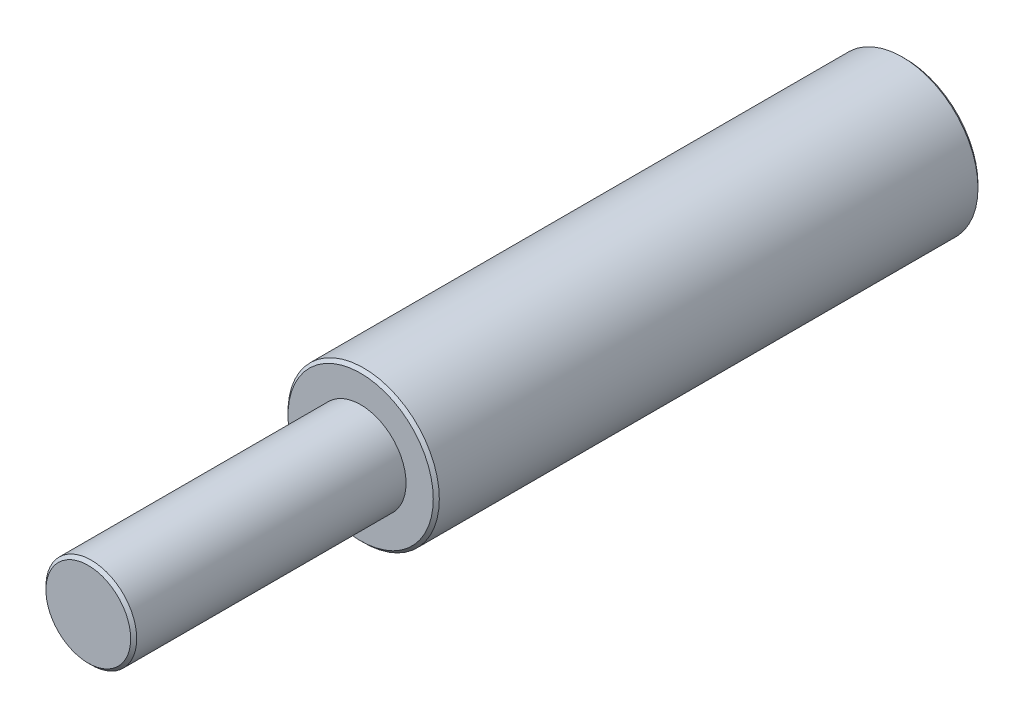
from build123d import *

# Parameters (mm, degrees)
SKETCH1_R           = 25
BOSS_EXTRUDE1_DEPTH = 180
SKETCH2_R           = 15
BOSS_EXTRUDE2_DEPTH = 90
CUT_EXTRUDE1_START  = -20
CUT_EXTRUDE1_DEPTH  = 120
CHAMFER1_SIZE       = 1
CUT_EXTRUDE2_START  = -10
SKETCH4_R           = 2.5
CUT_EXTRUDE2_DEPTH  = 10


with BuildPart() as part:
    # Sketch1 → Boss-Extrude1 (new body)
    with BuildSketch(Plane.XY):
        with Locations(Location((0, 0, 0), (0, 0, 180))):
            Circle(SKETCH1_R)
    extrude(amount=BOSS_EXTRUDE1_DEPTH)

    # Sketch2 → Boss-Extrude2 (add)
    with BuildSketch(Plane.XY.offset(180)):
        with Locations(Location((0, 0, 0), (0, 0, 180))):
            Circle(SKETCH2_R)
    extrude(amount=BOSS_EXTRUDE2_DEPTH)

    # Sketch3 → Cut-Extrude1 (cut)
    with BuildSketch(Plane(origin=(0, 0, 0), x_dir=(1, 0, 0), z_dir=(0, 1, 0)).offset(CUT_EXTRUDE1_START)):
        with BuildLine():
            Line((6, -84.229937471), (6, -134.229937471))
            ThreePointArc((6, -134.229937471), (0, -140.229937471), (-6, -134.229937471))
            Line((-6, -134.229937471), (-6, -84.229937471))
            ThreePointArc((-6, -84.229937471), (0, -78.229937471), (6, -84.229937471))
        make_face()
    extrude(amount=-CUT_EXTRUDE1_DEPTH, mode=Mode.SUBTRACT)

    # Chamfer1
    chamfer1_edges = [part.edges().sort_by_distance(p)[0] for p in [
        (25, 0, 0),
        (25, 0, 180),
        (15, 0, 270),
    ]]
    chamfer(chamfer1_edges, length=CHAMFER1_SIZE)

    # Sketch4 → Cut-Extrude2 (cut)
    with BuildSketch(Plane(origin=(0, 0, 0), x_dir=(0, 0, -1), z_dir=(1, 0, 0)).offset(CUT_EXTRUDE2_START)):
        with Locations((-211, 0)):
            Circle(SKETCH4_R)
    extrude(amount=-CUT_EXTRUDE2_DEPTH, mode=Mode.SUBTRACT)


solid = part.part
